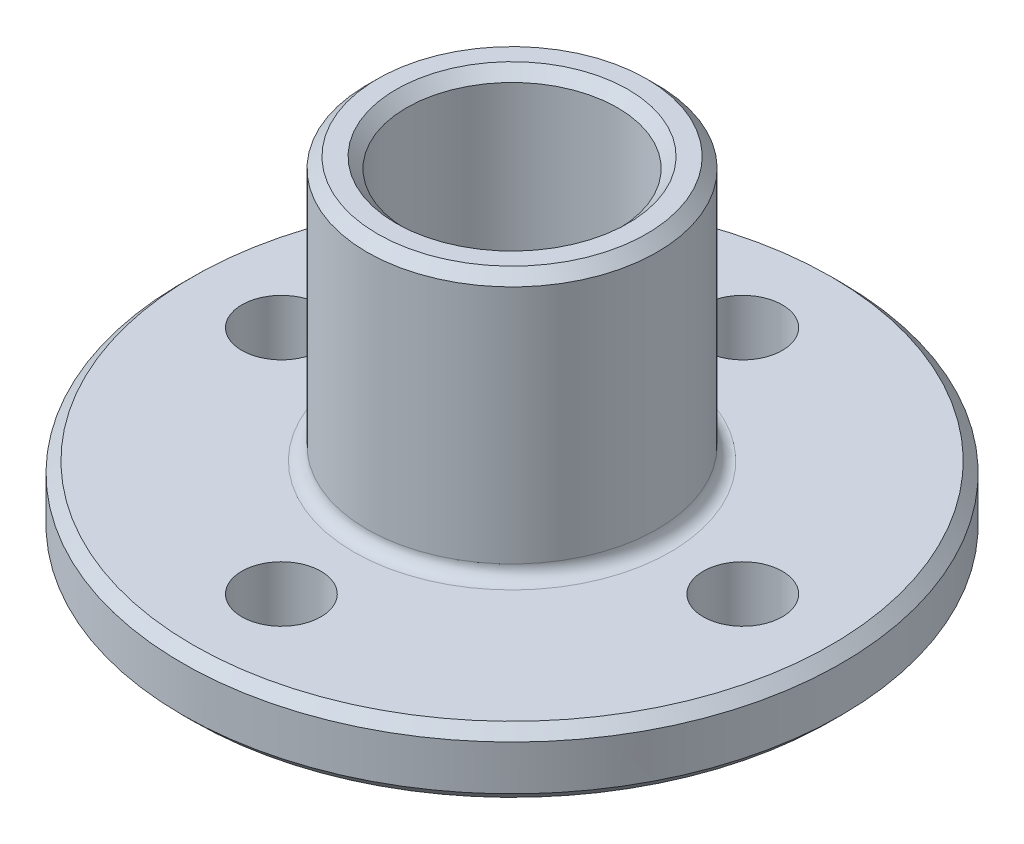
SolidWorks part; units mm, degrees
ref_plane "Front Plane" through (0, 0, 0) normal (0, 0, 1) x (1, 0, 0)
ref_plane "Top Plane" through (0, 0, 0) normal (0, 1, 0) x (1, 0, 0)
ref_plane "Right Plane" through (0, 0, 0) normal (1, 0, 0) x (0, 0, -1)
other "Configuration Table"
sketch "Sketch1" plane through (0, 0, 0) normal (0, 1, 0) x (1, 0, 0)
  circle A0 centre (0, 0) radius 25
  dimension "D1" = 50
extrude "Boss-Extrude2" add sketch "Sketch1" along normal blind 5
sketch "Sketch3" plane through (0, 0, 0) normal (0, 1, 0) x (1, 0, 0)
  line L0 (0, 0) -> (0, 17.5)
  line L1 (0, 0) -> (17.5, 0)
  line L2 (0, 0) -> (0, -17.5)
  line L3 (0, 0) -> (-17.5, 0)
  circle A0 centre (-17.5, 0) radius 3
  circle A1 centre (0, 17.5) radius 3
  circle A2 centre (17.5, 0) radius 3
  circle A3 centre (0, -17.5) radius 3
  point P9 (0, 0)
  point P17 (0, 0)
  dimension "D3" = 6
  dimension "D1" = 17.5
  dimension "D2" = 4
  dimension "D4" = 4
extrude "Cut-Extrude2" cut sketch "Sketch3" along normal blind 5 contours A0 | A1 | A2 | A3
sketch "Sketch4" plane through (0, 5, 0) normal (0, 1, 0) x (1, 0, 0)
  circle A0 centre (0, 0) radius 11
  circle A1 centre (0, 0) radius 8
  dimension "D1" = 22
  dimension "D2" = 16
extrude "Boss-Extrude3" add sketch "Sketch4" along normal blind 20
chamfer "Chamfer1" distance 0.8 angle 45 4 edges at (0, 25, 11) (0, 25, 8) (0, 5, 25) (0, 0, 25)
fillet "Fillet1" radius 1 1 edges at (0, 5, 11)
